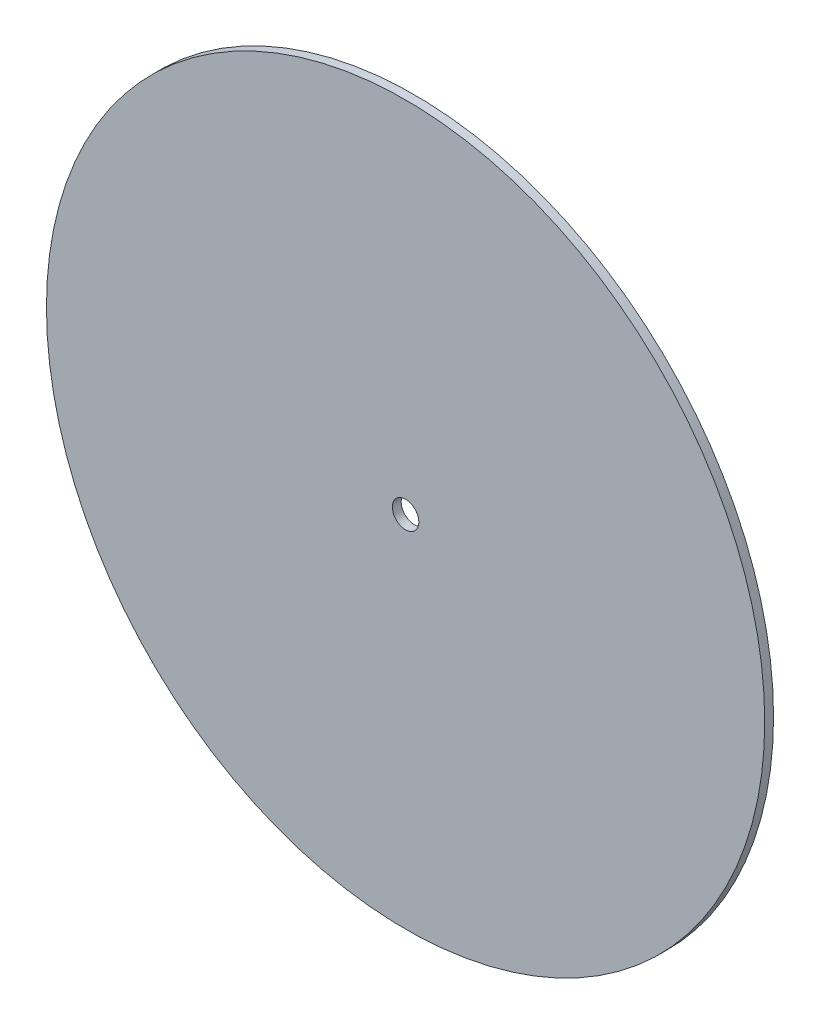
SolidWorks part; units mm, degrees
material "1023 碳钢板 (SS)"
ref_plane "前视基准面" through (0, 0, 0) normal (0, 0, 1) x (1, 0, 0)
ref_plane "上视基准面" through (0, 0, 0) normal (0, 1, 0) x (1, 0, 0)
ref_plane "右视基准面" through (0, 0, 0) normal (1, 0, 0) x (0, 0, -1)
sketch "草图1" plane through (0, 0, 0) normal (0, 0, 1) x (1, 0, 0)
  circle A0 centre (0, 0) radius 122.25
  circle A1 centre (0, 0) radius 4.5
  dimension "D1" = 244.5
  dimension "D2" = 9
extrude "凸台-拉伸1" add sketch "草图1" along normal blind 3
